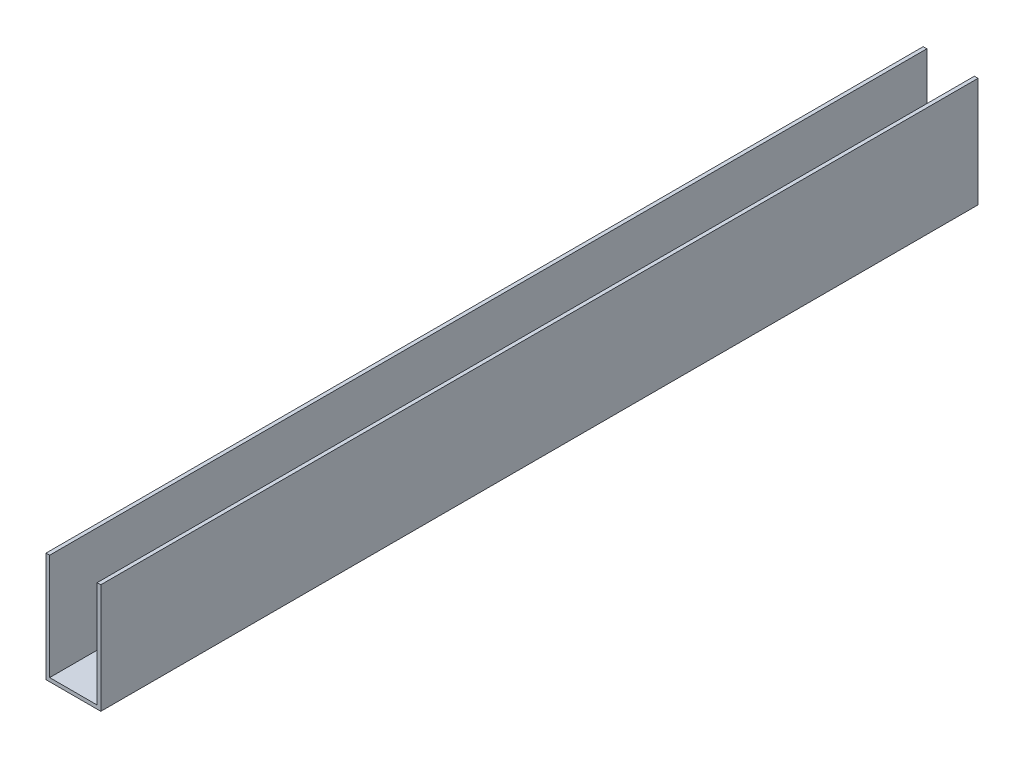
SolidWorks part; units mm, degrees
material "标准件"
ref_plane "前视基准面" through (0, 0, 0) normal (0, 0, 1) x (1, 0, 0)
ref_plane "上视基准面" through (0, 0, 0) normal (0, 1, 0) x (1, 0, 0)
ref_plane "右视基准面" through (0, 0, 0) normal (1, 0, 0) x (0, 0, -1)
sketch "草图1" plane through (0, 0, 0) normal (0, 0, 1) x (1, 0, 0)
  line L0 (0, 0) -> (0, 33.955) construction
  line L2 (-15, -30) -> (15, -30)
  line L3 (-15, -30) -> (-15, 30)
  line L4 (-15, 30) -> (15, 30)
  line L5 (15, -30) -> (15, 30)
  line L6 (-15, -30) -> (15, 30) construction
  line L7 (-15, 30) -> (15, -30) construction
  dimension "D1" = 30
  dimension "D2" = 60
extrude "凸台-拉伸1" add sketch "草图1" along normal mid plane 480
shell "抽壳1" thickness 2
